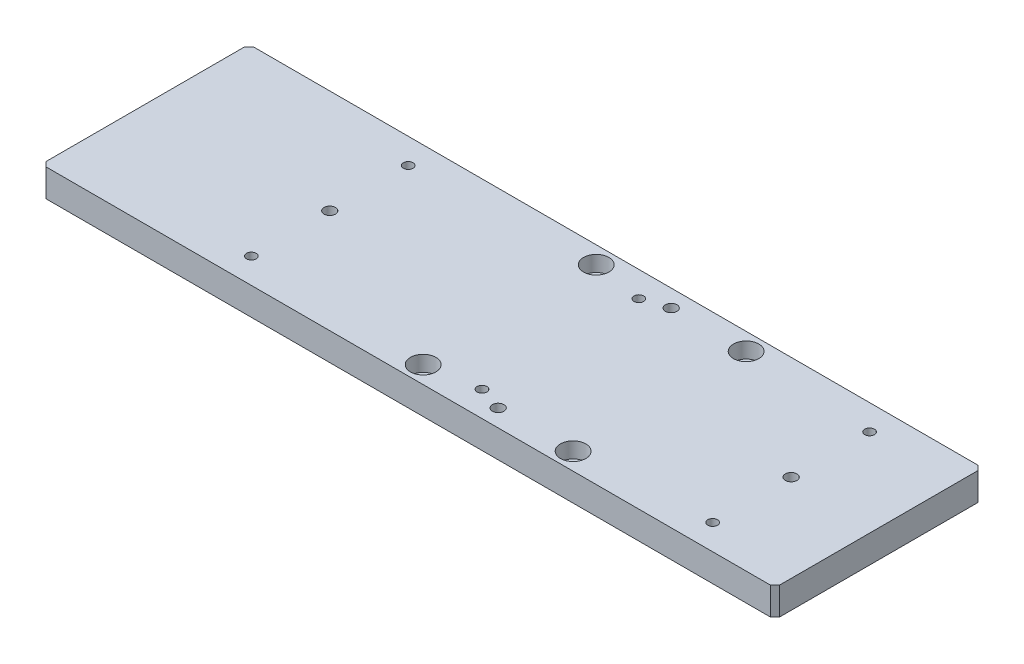
SolidWorks part; units mm, degrees
material "A6061"
ref_plane "前基準面" through (0, 0, 0) normal (0, 0, 1) x (1, 0, 0)
ref_plane "上基準面" through (0, 0, 0) normal (0, 1, 0) x (1, 0, 0)
ref_plane "右基準面" through (0, 0, 0) normal (1, 0, 0) x (0, 0, -1)
sketch "草图1" plane through (0, 0, 0) normal (0, 1, 0) x (1, 0, 0)
  line L1 (-159, -45) -> (159, -45)
  line L2 (-159, -45) -> (-159, 45)
  line L3 (-159, 45) -> (159, 45)
  line L4 (159, -45) -> (159, 45)
  line L5 (-159, -45) -> (159, 45) construction
  line L6 (-159, 45) -> (159, -45) construction
  point P0 (0, 0)
  dimension "D1" = 90
  dimension "D2" = 318
extrude "凸台-拉伸1" add sketch "草图1" along normal blind 12
hole_wizard "M6 六角圆柱头螺钉的柱形沉头孔1" positions "草图2" profile "草图3" counterbore size "M6" standard "GB" end condition through all
sketch "草图2" plane through (0, 12, 0) normal (0, 1, 0) x (1, 0, 0)
  line L0 (0, 0) -> (-179.0956, 0) construction
  line L1 (159, -45) -> (159, 45) construction
  point P0 (64, 37.5)
  point P7 (-1, 37.5)
  point P10 (-1, -37.5)
  point P11 (64, -37.5)
  dimension "D1" = 75
  dimension "D2" = 65
  dimension "D3" = 95
sketch "草图3" plane through (64, 12, -37.5) normal (1, 0, 0) x (0, 0, 1)
  line L0 (0, 0) -> (0, 12)
  line L1 (0, 12) -> (3.3, 12)
  line L3 (3.3, 12) -> (3.3, 6.8)
  line L4 (3.3, 6.8) -> (5.5, 6.8)
  line L5 (5.5, 6.8) -> (5.5, 0)
  line L7 (5.5, 0) -> (0, 0)
  line L11 (0, -6.35) -> (0, 107.95) construction
  dimension "通孔孔直径" = 6.6
  dimension "通孔孔深度" = 12
  dimension "柱形沉头孔直径" = 11
  dimension "柱形沉头孔深度" = 6.8
hole_wizard "M5 螺纹孔1" positions "草图4" profile "草图5" tap size "M5" standard "GB" end condition through all
sketch "草图4" plane through (0, 12, 0) normal (0, 1, 0) x (1, 0, 0)
  line L0 (0, 0) -> (183.6216, 0) construction
  line L1 (159, -45) -> (159, 45) construction
  point P0 (121, 34)
  point P3 (121, -34)
  point P14 (21, 34)
  point P15 (21, -34)
  point P17 (-79, 34)
  point P18 (-79, -34)
  dimension "D1" = 2
  dimension "D3" = 100
  dimension "D4" = 100
  dimension "D5" = 68
  dimension "D6" = 38
  dimension "D2" = 2
sketch "草图5" plane through (121, 12, -34) normal (1, 0, 0) x (0, 0, 1)
  line L0 (0, 0) -> (0, 12)
  line L1 (0, 12) -> (2.1, 12)
  line L2 (2.1, 12) -> (2.1, 0)
  line L5 (2.1, 0) -> (0, 0)
  line L11 (0, -6.35) -> (0, 107.95) construction
  dimension "通孔螺纹孔钻头直径" = 4.2
  dimension "通孔螺纹孔钻头深度" = 12
cosmetic thread "孔螺蚊线1" parameters "D2"=5
cosmetic thread "孔螺蚊线2" parameters "D2"=5
cosmetic thread "孔螺蚊线3" parameters "D2"=5
cosmetic thread "孔螺蚊线4" parameters "D2"=5
cosmetic thread "孔螺蚊线5" parameters "D2"=5
cosmetic thread "孔螺蚊线6" parameters "D2"=5
hole_wizard "Ø5.0mm 暗销孔1" positions "草图6" profile "草图7" hole size "Ø5.0" standard "GB"
sketch "草图6" plane through (0, 12, 0) normal (0, 1, 0) x (1, 0, 0)
  line L0 (121, 34) -> (121, -34) construction
  line L2 (-79, 34) -> (-79, -34) construction
  point P0 (121, 0)
  point P13 (-79, 0)
sketch "草图7" plane through (121, 12, 0) normal (1, 0, 0) x (0, 0, 1)
  line L0 (0, 0) -> (0, 7.5022)
  line L1 (0, 7.5022) -> (2.5, 6)
  line L2 (2.5, 6) -> (2.5, 0)
  line L5 (2.5, 0) -> (0, 0)
  line L10 (0, 7.5022) -> (-2.5, 6) construction
  line L11 (0, -6.35) -> (0, 107.95) construction
  dimension "孔直径" = 5
  dimension "孔深度" = 6
  dimension "导头角度" = 118
hole_wizard "Ø5.0mm 暗销孔2" positions "草图8" profile "草图9" hole size "Ø5.0" standard "GB"
sketch "草图8" plane through (0, 12, 0) normal (0, 1, 0) x (1, 0, 0)
  line L0 (-1, -37.5) -> (64, -37.5) construction
  line L3 (-1, 37.5) -> (64, 37.5) construction
  point P0 (31.5, -37.5)
  point P15 (31.5, 37.5)
sketch "草图9" plane through (31.5, 12, 37.5) normal (1, 0, 0) x (0, 0, 1)
  line L0 (0, 0) -> (0, 6.5022)
  line L1 (0, 6.5022) -> (2.5, 5)
  line L2 (2.5, 5) -> (2.5, 0)
  line L5 (2.5, 0) -> (0, 0)
  line L10 (0, 6.5022) -> (-2.5, 5) construction
  line L11 (0, -6.35) -> (0, 107.95) construction
  dimension "孔直径" = 5
  dimension "孔深度" = 5
  dimension "导头角度" = 118
chamfer "倒角1" distance 2 angle 45 4 edges at (-159, 6, 45) (-159, 6, -45) (159, 6, -45) (159, 6, 45)
